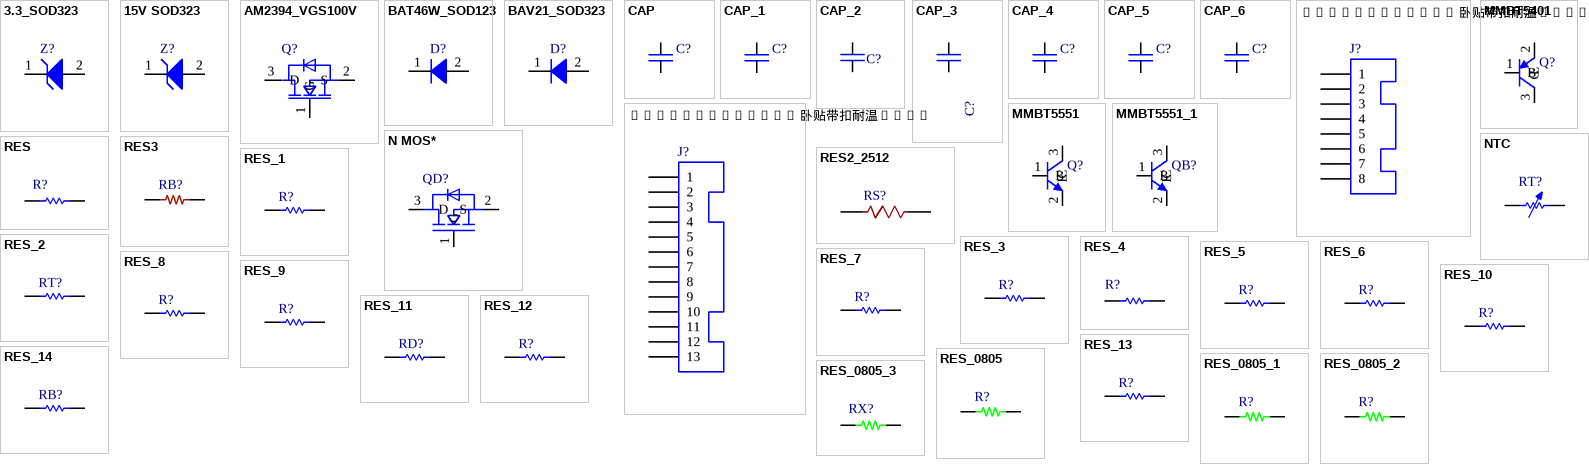
[diagram p0: symbols 3.3_SOD323 to RES_0805_3]
# Altium schematic symbol library MISC82749.SCHLIB: 46 symbols
Pins are listed as number, name and electrical type; pins without a type are passive.


## 3.3_SOD323
designator Z?
SMD zener diode
footprint SOD323A (SMD diode)
pins: 1 A, 2 K

## 15V SOD323
designator Z?
SMD zener diode
footprint SOD323A (SMD diode)
pins: 1 A, 2 K

## AM2394_VGS100V
designator Q?
SMD N MOS_VGS100V
footprint SOT23-3L (SMD MOSFET)
footprint SOT23-3 (SMD IC/MOS*)
pins: 1 G, 2 S, 3 D

## BAT46W_SOD123
designator D?
SMD diode
footprint SOD123A (SMD diode)
footprint SOD123 (SMD diode)
pins: 1 A, 2 K

## BAV21_SOD323
designator D?
SMD diode
footprint SOD323A (SMD diode)
pins: 1 A, 2 K

## CAP
designator C?
SMD capacitor
footprint C0402A (SMD capacitor)
footprint C0603A (SMD capacitor)
footprint C0402L (SMD resistor)
footprint C0805A (SMD capacitor)
footprint C1206A (SMD capacitor)
footprint C0603L (SMD J capacitor)
footprint C0805L (SMD capacitor)
footprint C0603M (SMD capacitor)
pins: 1, 2

## CAP_1
designator C?
SMD capacitor
footprint C0402A (SMD capacitor)
footprint C0603A (SMD capacitor)
footprint C0402L (SMD resistor)
footprint C0805A (SMD capacitor)
footprint C1206A (SMD capacitor)
footprint C0603L (SMD J capacitor)
footprint C0805L (SMD capacitor)
footprint C0603M (SMD capacitor)
pins: 1, 2

## CAP_2
designator C?
SMD capacitor
footprint C0402A (SMD capacitor)
footprint C0603A (SMD capacitor)
footprint C0402L (SMD resistor)
footprint C0805A (SMD capacitor)
footprint C1206A (SMD capacitor)
footprint C0603L (SMD J capacitor)
footprint C0805L (SMD capacitor)
footprint C0603M (SMD capacitor)
pins: 1, 2

## CAP_3
designator C?
SMD capacitor
footprint C0402A (SMD capacitor)
footprint C0603A (SMD capacitor)
footprint C0402L (SMD resistor)
footprint C0805A (SMD capacitor)
footprint C1206A (SMD capacitor)
footprint C0603L (SMD J capacitor)
footprint C0805L (SMD capacitor)
footprint C0603M (SMD capacitor)
pins: 1, 2

## CAP_4
designator C?
SMD capacitor
footprint C0402A (SMD capacitor)
footprint C0603A (SMD capacitor)
footprint C0402L (SMD resistor)
footprint C0805A (SMD capacitor)
footprint C1206A (SMD capacitor)
footprint C0603L (SMD J capacitor)
footprint C0805L (SMD capacitor)
footprint C0603M (SMD capacitor)
pins: 1, 2

## CAP_5
designator C?
SMD capacitor
footprint C0402A (SMD capacitor)
footprint C0603A (SMD capacitor)
footprint C0402L (SMD resistor)
footprint C0805A (SMD capacitor)
footprint C1206A (SMD capacitor)
footprint C0603L (SMD J capacitor)
footprint C0805L (SMD capacitor)
footprint C0603M (SMD capacitor)
pins: 1, 2

## CAP_6
designator C?
SMD capacitor
footprint C0402A (SMD capacitor)
footprint C0603A (SMD capacitor)
footprint C0402L (SMD resistor)
footprint C0805A (SMD capacitor)
footprint C1206A (SMD capacitor)
footprint C0603L (SMD J capacitor)
footprint C0805L (SMD capacitor)
footprint C0603M (SMD capacitor)
pins: 1, 2

## HY2.0WT-8A/P 卧贴带扣耐温260℃
designator J?
horizontal SMD latched connector, 260℃ heat-resistant
footprint HY2.0WT-8A/P 卧贴带扣耐温260℃ (horizontal SMD connector)
footprint 2.0-8PIN直针带扣连接器 (upright plug-in connector)
pins: 1, 2, 3, 4, 5, 6, 7, 8

## HY2.0WT-13A/P 卧贴带扣耐温260℃
designator J?
horizontal SMD latched connector, 260℃ heat-resistant
footprint 2-13P 卧贴带扣耐温260℃ (horizontal SMD connector)
footprint 2.0-13PIN直针带扣连接器 (upright plug-in connector)
pins: 1, 2, 3, 4, 5, 6, 7, 8, 9, 10, 11, 12, 13

## MMBT5401
designator Q?
SMD transistor
footprint SOT23-3 (SMD IC/MOS*)
footprint SOT23-3L (SMD MOSFET)
footprint SOT23-3 (SMD IC/MOS*)
pins: 1 B, 2 E, 3 C

## MMBT5551
designator Q?
SMD transistor
footprint SOT23-3 (SMD IC/MOS*)
footprint SOT23-3L (SMD MOSFET)
pins: 1 B, 2 E, 3 C

## MMBT5551_1
designator QB?
SMD transistor
footprint SOT23-3 (SMD IC/MOS*)
footprint SOT23-3L (SMD MOSFET)
pins: 1 B, 2 E, 3 C

## N MOS*
designator QD?
SMD MOSFET
footprint TO-252
footprint TO-252-DFN
footprint SOP-8L(T3p)
footprint DFN5X6(T3p) (SMD MOSFET (non-standard))
footprint TO-263-TOLL
footprint DFN-3x3L8(T3P) (SMD MOSFET)
footprint TOLL_123 (SMD MOSFET)
footprint TOLL_GSD (SMD MOSFET)
pins: 1 G, 2 S, 3 D

## NTC
designator RT?
SMD thermistor
footprint R0603A (SMD resistor)
footprint R0402A (SMD resistor)
footprint RT2.3X1-2 (wire-lead NTC)
footprint R0603L (SMD resistor)
footprint R0603m (SMD resistor)
footprint RT2.3X1.2-2 (wire-lead NTC)
pins: 1, 2

## RES
designator R?
SMD resistor
footprint R0603A (SMD resistor)
footprint R0201A
footprint R0402A (SMD resistor)
footprint R0603m (SMD resistor)
footprint R0805A (SMD resistor)
footprint R0402L (SMD resistor)
footprint RES0603 (CAP0402)
footprint R0603L (SMD resistor)
footprint R0805L (SMD resistor)
footprint R0805M (SMD resistor)
footprint R1206A (SMD resistor)
pins: 1, 2

## RES2_2512
designator RS?
SMD alloy resistor
footprint R2512L (SMD resistor)
pins: 1, 2

## RES3
designator RB?
alloy SMD resistor
footprint R1206A
pins: 1, 2

## RES_1
designator R?
SMD resistor
footprint R0603A (SMD resistor)
footprint R0201A
footprint R0402A (SMD resistor)
footprint R0603m (SMD resistor)
footprint R0805A (SMD resistor)
footprint R0402L (SMD resistor)
footprint RES0603 (CAP0402)
footprint R0603L (SMD resistor)
footprint R0805L (SMD resistor)
footprint R0805M (SMD resistor)
footprint R1206A (SMD resistor)
pins: 1, 2

## RES_2
designator RT?
SMD resistor
footprint R0603A (SMD resistor)
footprint R0201A
footprint R0402A (SMD resistor)
footprint R0603m (SMD resistor)
footprint R0805A (SMD resistor)
footprint R0402L (SMD resistor)
footprint RES0603 (CAP0402)
footprint R0603L (SMD resistor)
footprint R0805L (SMD resistor)
footprint R0805M (SMD resistor)
footprint R1206A (SMD resistor)
pins: 1, 2

## RES_3
designator R?
SMD resistor
footprint R0603A (SMD resistor)
footprint R0201A
footprint R0402A (SMD resistor)
footprint R0603m (SMD resistor)
footprint R0805A (SMD resistor)
footprint R0402L (SMD resistor)
footprint RES0603 (CAP0402)
footprint R0603L (SMD resistor)
footprint R0805L (SMD resistor)
footprint R0805M (SMD resistor)
footprint R1206A (SMD resistor)
pins: 1, 2

## RES_4
designator R?
SMD resistor
footprint R0603A (SMD resistor)
footprint R0201A
footprint R0402A (SMD resistor)
footprint R0603m (SMD resistor)
footprint R0805A (SMD resistor)
footprint R0402L (SMD resistor)
footprint RES0603 (CAP0402)
footprint R0603L (SMD resistor)
footprint R0805L (SMD resistor)
footprint R0805M (SMD resistor)
footprint R1206A (SMD resistor)
pins: 1, 2

## RES_5
designator R?
SMD resistor
footprint R0603A (SMD resistor)
footprint R0201A
footprint R0402A (SMD resistor)
footprint R0603m (SMD resistor)
footprint R0805A (SMD resistor)
footprint R0402L (SMD resistor)
footprint RES0603 (CAP0402)
footprint R0603L (SMD resistor)
footprint R0805L (SMD resistor)
footprint R0805M (SMD resistor)
footprint R1206A (SMD resistor)
pins: 1, 2

## RES_6
designator R?
SMD resistor
footprint R0603A (SMD resistor)
footprint R0201A
footprint R0402A (SMD resistor)
footprint R0603m (SMD resistor)
footprint R0805A (SMD resistor)
footprint R0402L (SMD resistor)
footprint RES0603 (CAP0402)
footprint R0603L (SMD resistor)
footprint R0805L (SMD resistor)
footprint R0805M (SMD resistor)
footprint R1206A (SMD resistor)
pins: 1, 2

## RES_7
designator R?
SMD resistor
footprint R0603A (SMD resistor)
footprint R0201A
footprint R0402A (SMD resistor)
footprint R0603m (SMD resistor)
footprint R0805A (SMD resistor)
footprint R0402L (SMD resistor)
footprint RES0603 (CAP0402)
footprint R0603L (SMD resistor)
footprint R0805L (SMD resistor)
footprint R0805M (SMD resistor)
footprint R1206A (SMD resistor)
pins: 1, 2

## RES_8
designator R?
SMD resistor
footprint R0603A (SMD resistor)
footprint R0201A
footprint R0402A (SMD resistor)
footprint R0603m (SMD resistor)
footprint R0805A (SMD resistor)
footprint R0402L (SMD resistor)
footprint RES0603 (CAP0402)
footprint R0603L (SMD resistor)
footprint R0805L (SMD resistor)
footprint R0805M (SMD resistor)
footprint R1206A (SMD resistor)
pins: 1, 2

## RES_9
designator R?
SMD resistor
footprint R0603A (SMD resistor)
footprint R0201A
footprint R0402A (SMD resistor)
footprint R0603m (SMD resistor)
footprint R0805A (SMD resistor)
footprint R0402L (SMD resistor)
footprint RES0603 (CAP0402)
footprint R0603L (SMD resistor)
footprint R0805L (SMD resistor)
footprint R0805M (SMD resistor)
footprint R1206A (SMD resistor)
pins: 1, 2

## RES_10
designator R?
SMD resistor
footprint R0603A (SMD resistor)
footprint R0201A
footprint R0402A (SMD resistor)
footprint R0603m (SMD resistor)
footprint R0805A (SMD resistor)
footprint R0402L (SMD resistor)
footprint RES0603 (CAP0402)
footprint R0603L (SMD resistor)
footprint R0805L (SMD resistor)
footprint R0805M (SMD resistor)
footprint R1206A (SMD resistor)
pins: 1, 2

## RES_11
designator RD?
SMD resistor
footprint R0603A (SMD resistor)
footprint R0201A
footprint R0402A (SMD resistor)
footprint R0603m (SMD resistor)
footprint R0805A (SMD resistor)
footprint R0402L (SMD resistor)
footprint RES0603 (CAP0402)
footprint R0603L (SMD resistor)
footprint R0805L (SMD resistor)
footprint R0805M (SMD resistor)
footprint R1206A (SMD resistor)
pins: 1, 2

## RES_12
designator R?
SMD resistor
footprint R0603A (SMD resistor)
footprint R0201A
footprint R0402A (SMD resistor)
footprint R0603m (SMD resistor)
footprint R0805A (SMD resistor)
footprint R0402L (SMD resistor)
footprint RES0603 (CAP0402)
footprint R0603L (SMD resistor)
footprint R0805L (SMD resistor)
footprint R0805M (SMD resistor)
footprint R1206A (SMD resistor)
pins: 1, 2

## RES_13
designator R?
SMD resistor
footprint R0603A (SMD resistor)
footprint R0201A
footprint R0402A (SMD resistor)
footprint R0603m (SMD resistor)
footprint R0805A (SMD resistor)
footprint R0402L (SMD resistor)
footprint RES0603 (CAP0402)
footprint R0603L (SMD resistor)
footprint R0805L (SMD resistor)
footprint R0805M (SMD resistor)
footprint R1206A (SMD resistor)
pins: 1, 2

## RES_14
designator RB?
SMD resistor
footprint R0603A (SMD resistor)
footprint R0201A
footprint R0402A (SMD resistor)
footprint R0603m (SMD resistor)
footprint R0805A (SMD resistor)
footprint R0402L (SMD resistor)
footprint RES0603 (CAP0402)
footprint R0603L (SMD resistor)
footprint R0805L (SMD resistor)
footprint R0805M (SMD resistor)
footprint R1206A (SMD resistor)
pins: 1, 2

## RES_0805
designator R?
SMD resistor
footprint R0805L (SMD resistor)
pins: 1, 2

## RES_0805_1
designator R?
SMD resistor
footprint R0805L (SMD resistor)
pins: 1, 2

## RES_0805_2
designator R?
SMD resistor
footprint R0805L (SMD resistor)
pins: 1, 2

## RES_0805_3
designator RX?
SMD resistor
footprint R0805L (SMD resistor)
pins: 1, 2

## RS3M
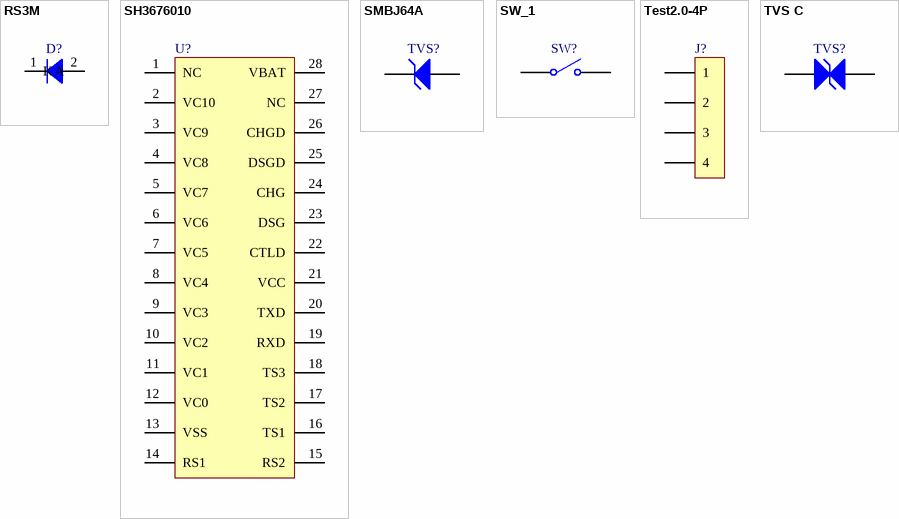
[diagram p1: symbols RS3M to TVS C]
## RS3M
designator D?
SMD diode
footprint SMB A (SMD diode)
pins: 1 A, 2 K

## SH3676010
designator U?
footprint TSSOP-28L
footprint TSSOP-28L(PIN间距0.65mm) (SMD IC)
pins: 1 NC, 2 VC10, 3 VC9, 4 VC8, 5 VC7, 6 VC6, 7 VC5, 8 VC4, 9 VC3, 10 VC2, 11 VC1, 12 VC0, 13 VSS, 14 RS1, 15 RS2, 16 TS1, 17 TS2, 18 TS3, 19 RXD, 20 TXD, 21 VCC, 22 CTLD, 23 DSG, 24 CHG, 25 DSGD, 26 CHGD, 27 NC, 28 VBAT

## SMBJ64A
designator TVS?
SMD diode (ESD and surge protection)
footprint SMB(DO-214AA) (SMD diode)
footprint SMB A (SMD diode)
pins: 1 A, 2 K

## SW_1
designator SW?
soft-touch switch
footprint RT2.3X1.2-2 (wire-lead NTC)
pins: 1 COMMON, 2 NO

## Test2.0-4P
designator J?
test socket
footprint Test2.0-4P (test socket 2.0mm)
pins: 1, 2, 3, 4

## TVS C
designator TVS?
SMD diode (ESD and surge protection)
footprint SMC A-TVS(DO-214AB) (SMD diode)
footprint SMC A_AK(DO-214AB) (SMD diode)
footprint SMC_MDO-214AB) (SMD diode)
pins: 1 A, 2 K